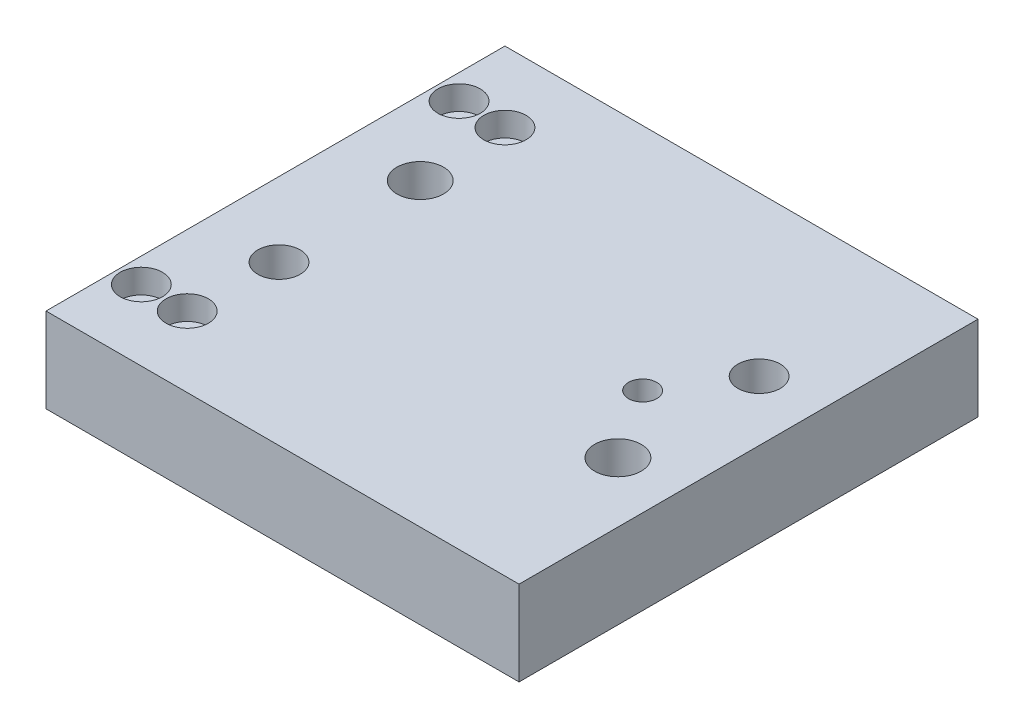
SolidWorks part; units mm, degrees
material "A6061"
ref_plane "前基準面" through (0, 0, 0) normal (0, 0, 1) x (1, 0, 0)
ref_plane "上基準面" through (0, 0, 0) normal (0, 1, 0) x (1, 0, 0)
ref_plane "右基準面" through (0, 0, 0) normal (1, 0, 0) x (0, 0, -1)
sketch "草图1" plane through (0, 0, 0) normal (0, 1, 0) x (1, 0, 0)
  line L0 (0, 0) -> (48.7516, 0) construction
  line L1 (-33.5, -32.5) -> (33.5, -32.5)
  line L2 (-33.5, -32.5) -> (-33.5, 32.5)
  line L3 (-33.5, 32.5) -> (33.5, 32.5)
  line L4 (33.5, -32.5) -> (33.5, 32.5)
  line L5 (-33.5, -32.5) -> (33.5, 32.5) construction
  line L6 (-33.5, 32.5) -> (33.5, -32.5) construction
  circle A0 centre (18.5, 0) radius 2
  point P0 (0, 0)
  dimension "D3" = 4
  dimension "D4" = 15
  dimension "D1" = 67
  dimension "D2" = 65
extrude "凸台-拉伸1" add sketch "草图1" along normal mid plane 12
sketch "草图2" plane through (0, -6, 0) normal (0, 1, 0) x (1, 0, 0)
  line L0 (0, 39.8262) -> (0, 0) construction
  line L1 (0, 0) -> (-41.7993, 0) construction
  line L3 (25, -10) -> (-23, -10) construction
  line L4 (25, -10) -> (25, 10) construction
  line L5 (25, 10) -> (-23, 10) construction
  line L6 (-23, -10) -> (-23, 10) construction
  line L7 (33.5, -32.5) -> (33.5, 32.5) construction
  point P0 (-23, 10)
  point P19 (25, -10)
  dimension "D1" = 20
  dimension "D2" = 48
  dimension "D3" = 8.5
sketch "草图4" plane through (0, 6, 0) normal (0, 1, 0) x (1, 0, 0)
  line L0 (-26.75, 25.9571) -> (-26.75, -30) construction
  line L1 (-26.75, -30) -> (-47.4826, -30) construction
  line L2 (0, 0) -> (-51.4415, 0) construction
  line L4 (-33.5, 32.5) -> (-33.5, -32.5) construction
  point P0 (-30, -22.5)
  point P10 (-30, -37.5)
  point P11 (-23.5, -37.5)
  point P12 (-23.5, -22.5)
  point P21 (-23.5, 22.5)
  point P22 (-23.5, 37.5)
  point P23 (-30, 37.5)
  point P24 (-30, 22.5)
  dimension "D1" = 6.5
  dimension "D2" = 15
  dimension "D3" = 60
  dimension "D4" = 3.5
sketch "草图6" plane through (0, 6, 0) normal (0, 1, 0) x (1, 0, 0)
  line L0 (33.5, -32.5) -> (23.5, -32.5)
  line L5 (33.5, -32.5) -> (33.5, -7.5)
  line L6 (0, 56.6769) -> (0, 0) construction
  line L7 (0, 0) -> (-35.7167, 0) construction
  line L16 (23.5, 32.5) -> (23.5, 12.5)
  line L17 (33.5, 7.5) -> (28.5, 7.5)
  line L18 (33.5, 32.5) -> (33.5, 7.5)
  line L19 (33.5, 32.5) -> (23.5, 32.5)
  line L20 (33.5, -32.5) -> (33.5, 32.5) construction
  line L21 (33.5, -7.5) -> (28.5, -7.5)
  line L22 (23.5, -32.5) -> (23.5, -12.5)
  arc A3 (28.5, 7.5) -> (23.5, 12.5) centre (28.5, 12.5) cw
  arc A4 (28.5, -7.5) -> (23.5, -12.5) centre (28.5, -12.5) ccw
  dimension "D1" = 25
  dimension "D3" = 5
  dimension "D2" = 10
sketch "草图9" plane through (0, 6, 0) normal (0, 1, 0) x (1, 0, 0)
  line L0 (18.5, 0) -> (18.5, -49.0461) construction
  line L1 (-21.5, 42.5) -> (-16.5, 27.5)
  line L2 (-21.5, -42.5) -> (-21.5, 42.5)
  line L3 (-16.5, -27.5) -> (-21.5, -42.5)
  line L4 (3.5, 47.5) -> (33.5, 47.5)
  line L5 (3.5, -47.5) -> (33.5, -47.5)
  line L9 (33.5, -32.5) -> (33.5, 32.5)
  line L12 (33.5, 32.5) -> (-33.5, 32.5)
  line L13 (-33.5, 32.5) -> (-33.5, -32.5)
  line L14 (-33.5, -32.5) -> (33.5, -32.5)
  line L17 (33.5, -32.5) -> (33.5, 32.5)
  arc A0 (3.5, 47.5) -> (-16.5, 27.5) centre (-16.5, 47.5) cw
  arc A1 (-16.5, -27.5) -> (3.5, -47.5) centre (-16.5, -47.5) cw
  circle A6 centre (18.5, 0) radius 2 construction
  circle A7 centre (18.5, 0) radius 2
  dimension "D1" = 0
hole_wizard "M3 六角圆柱头螺钉的柱形沉头孔1" positions "草图4" profile "草图5" counterbore size "M3" standard "GB" end condition through all
sketch "草图5" plane through (-30, 6, 22.5) normal (1, 0, 0) x (0, 0, 1)
  line L0 (0, 0) -> (0, 12)
  line L1 (0, 12) -> (1.7, 12)
  line L3 (1.7, 12) -> (1.7, 3.4)
  line L4 (1.7, 3.4) -> (3, 3.4)
  line L5 (3, 3.4) -> (3, 0)
  line L7 (3, 0) -> (0, 0)
  line L11 (0, -6.35) -> (0, 107.95) construction
  dimension "通孔孔直径" = 3.4
  dimension "通孔孔深度" = 12
  dimension "柱形沉头孔直径" = 6
  dimension "柱形沉头孔深度" = 3.4
hole_wizard "M6 六角圆柱头螺钉的柱形沉头孔1" positions "草图2" profile "草图3" counterbore size "M6" standard "GB" end condition through all
sketch "草图3" plane through (-23, -6, -10) normal (1, 0, 0) x (0, 0, -1)
  line L0 (0, 0) -> (0, 12)
  line L1 (0, 12) -> (3.3, 12)
  line L3 (3.3, 12) -> (3.3, 6.8)
  line L4 (3.3, 6.8) -> (5.5, 6.8)
  line L5 (5.5, 6.8) -> (5.5, 0)
  line L7 (5.5, 0) -> (0, 0)
  line L11 (0, -6.35) -> (0, 107.95) construction
  dimension "通孔孔直径" = 6.6
  dimension "通孔孔深度" = 12
  dimension "柱形沉头孔直径" = 11
  dimension "柱形沉头孔深度" = 6.8
hole_wizard "Ø6.0mm 暗销孔1" positions "草图7" profile "草图8" hole size "Ø6.0" standard "GB" end condition up to next
sketch "草图7" plane through (0, -6, 0) normal (0, -1, 0) x (-1, 0, 0)
  line L0 (23, 10) -> (23, -10) construction
  line L1 (23, -10) -> (-25, -10) construction
  line L2 (-25, -10) -> (-25, 10) construction
  line L3 (-25, 10) -> (23, 10) construction
  point P0 (-25, 10)
  point P5 (23, -10)
  point P19 (23, -10)
sketch "草图8" plane through (25, -6, -10) normal (1, 0, 0) x (0, 0, -1)
  line L0 (0, 0) -> (0, 12)
  line L1 (0, 12) -> (3, 12)
  line L2 (3, 12) -> (3, 0)
  line L5 (3, 0) -> (0, 0)
  line L11 (0, -6.35) -> (0, 107.95) construction
  dimension "通孔孔直径" = 6
  dimension "通孔孔深度" = 12
